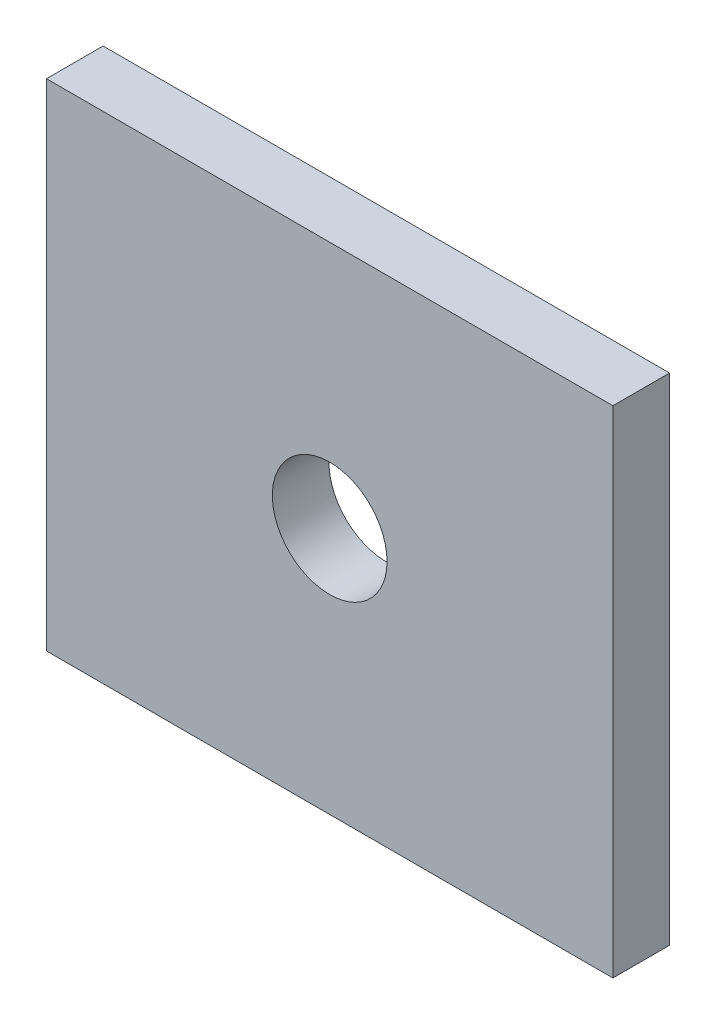
SolidWorks part; units mm, degrees
ref_plane "前视基准面" through (0, 0, 0) normal (0, 0, 1) x (1, 0, 0)
ref_plane "上视基准面" through (0, 0, 0) normal (0, 1, 0) x (1, 0, 0)
ref_plane "右视基准面" through (0, 0, 0) normal (1, 0, 0) x (0, 0, -1)
other "Configuration Table"
sketch "草图1" plane through (0, 0, 0) normal (0, 0, 1) x (1, 0, 0)
  line L0 (-40, -35) -> (40, -35)
  line L1 (40, -35) -> (40, 35)
  line L2 (40, 35) -> (-40, 35)
  line L3 (-40, 35) -> (-40, -35)
  point P0 (0, 0)
  dimension "D1" = 40
  dimension "D2" = 80
  dimension "D3" = 35
  dimension "D4" = 70
extrude "凸台-拉伸1" add sketch "草图1" against normal mid plane 8
sketch "草图2" plane through (0, 0, 0) normal (0, 0, 1) x (1, 0, 0)
  circle A0 centre (0, 0) radius 8.1
  point P0 (0, 0)
  dimension "D1" = 16.2
extrude "切除-拉伸1" cut sketch "草图2" against normal mid plane 28
